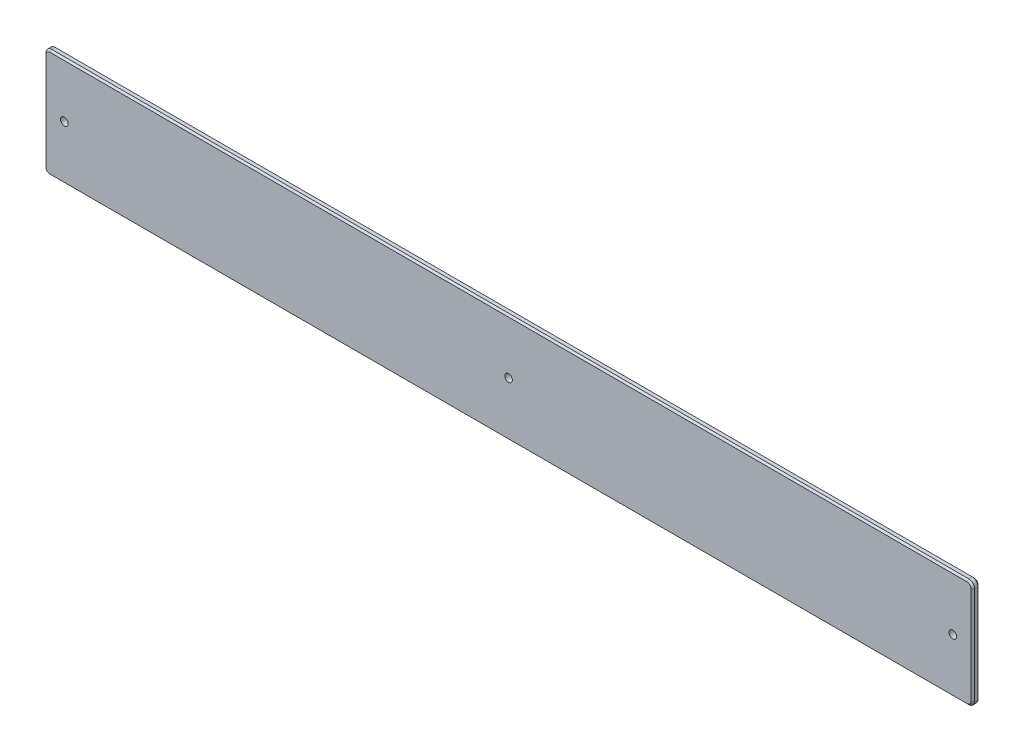
from build123d import *

# Parameters (mm, degrees)
SKETCH1_W           = 810
SKETCH1_H           = 95
BOSS_EXTRUDE1_DEPTH = 6
FILLET1_R           = 5
CHAMFER1_SIZE       = 1.5
CUT_EXTRUDE1_REACH  = 409.82
SKETCH2_R           = 3.3


with BuildPart() as part:
    # Sketch1 → Boss-Extrude1 (new body)
    with BuildSketch(Plane.XY):
        Rectangle(SKETCH1_W, SKETCH1_H)
    extrude(amount=BOSS_EXTRUDE1_DEPTH)

    # Fillet1
    fillet1_edges = [part.edges().sort_by_distance(p)[0] for p in [
        (-405, 47.5, 3),
        (405, 47.5, 3),
        (405, -47.5, 3),
        (-405, -47.5, 3),
    ]]
    fillet(fillet1_edges, radius=FILLET1_R)

    # Chamfer1
    chamfer1_edges = [part.edges().sort_by_distance(p)[0] for p in [
        (0, 47.5, 0),
        (0, 47.5, 6),
        (-405, 0, 0),
        (405, 0, 0),
        (0, -47.5, 0),
        (-403.535533906, 46.035533906, 0),
        (-403.535533906, -46.035533906, 0),
        (403.535533906, -46.035533906, 0),
        (403.535533906, 46.035533906, 0),
        (405, 0, 6),
        (-405, 0, 6),
        (0, -47.5, 6),
        (-403.535533906, 46.035533906, 6),
        (-403.535533906, -46.035533906, 6),
        (403.535533906, -46.035533906, 6),
        (403.535533906, 46.035533906, 6),
    ]]
    chamfer(chamfer1_edges, length=CHAMFER1_SIZE)

    # Sketch2 → Cut-Extrude1 (cut, up to next)
    with BuildSketch(Plane.XY.offset(6), mode=Mode.PRIVATE) as cut_extrude1_sk1:
        with Locations((-387.5, 0)):
            Circle(SKETCH2_R)
    cut_extrude1_tool1 = extrude(cut_extrude1_sk1.sketch, amount=-CUT_EXTRUDE1_REACH, mode=Mode.PRIVATE) & part.part
    # Sketch2 → Cut-Extrude1 (cut, up to next)
    with BuildSketch(Plane.XY.offset(6), mode=Mode.PRIVATE) as cut_extrude1_sk2:
        Circle(SKETCH2_R)
    cut_extrude1_tool2 = extrude(cut_extrude1_sk2.sketch, amount=-CUT_EXTRUDE1_REACH, mode=Mode.PRIVATE) & part.part
    # Sketch2 → Cut-Extrude1 (cut, up to next)
    with BuildSketch(Plane.XY.offset(6), mode=Mode.PRIVATE) as cut_extrude1_sk3:
        with Locations((387.5, 0)):
            Circle(SKETCH2_R)
    cut_extrude1_tool3 = extrude(cut_extrude1_sk3.sketch, amount=-CUT_EXTRUDE1_REACH, mode=Mode.PRIVATE) & part.part
    add(cut_extrude1_tool1.solids().sort_by_distance((-387.5, 0, 6))[0], mode=Mode.SUBTRACT)
    add(cut_extrude1_tool2.solids().sort_by_distance((0, 0, 6))[0], mode=Mode.SUBTRACT)
    add(cut_extrude1_tool3.solids().sort_by_distance((387.5, 0, 6))[0], mode=Mode.SUBTRACT)


solid = part.part
